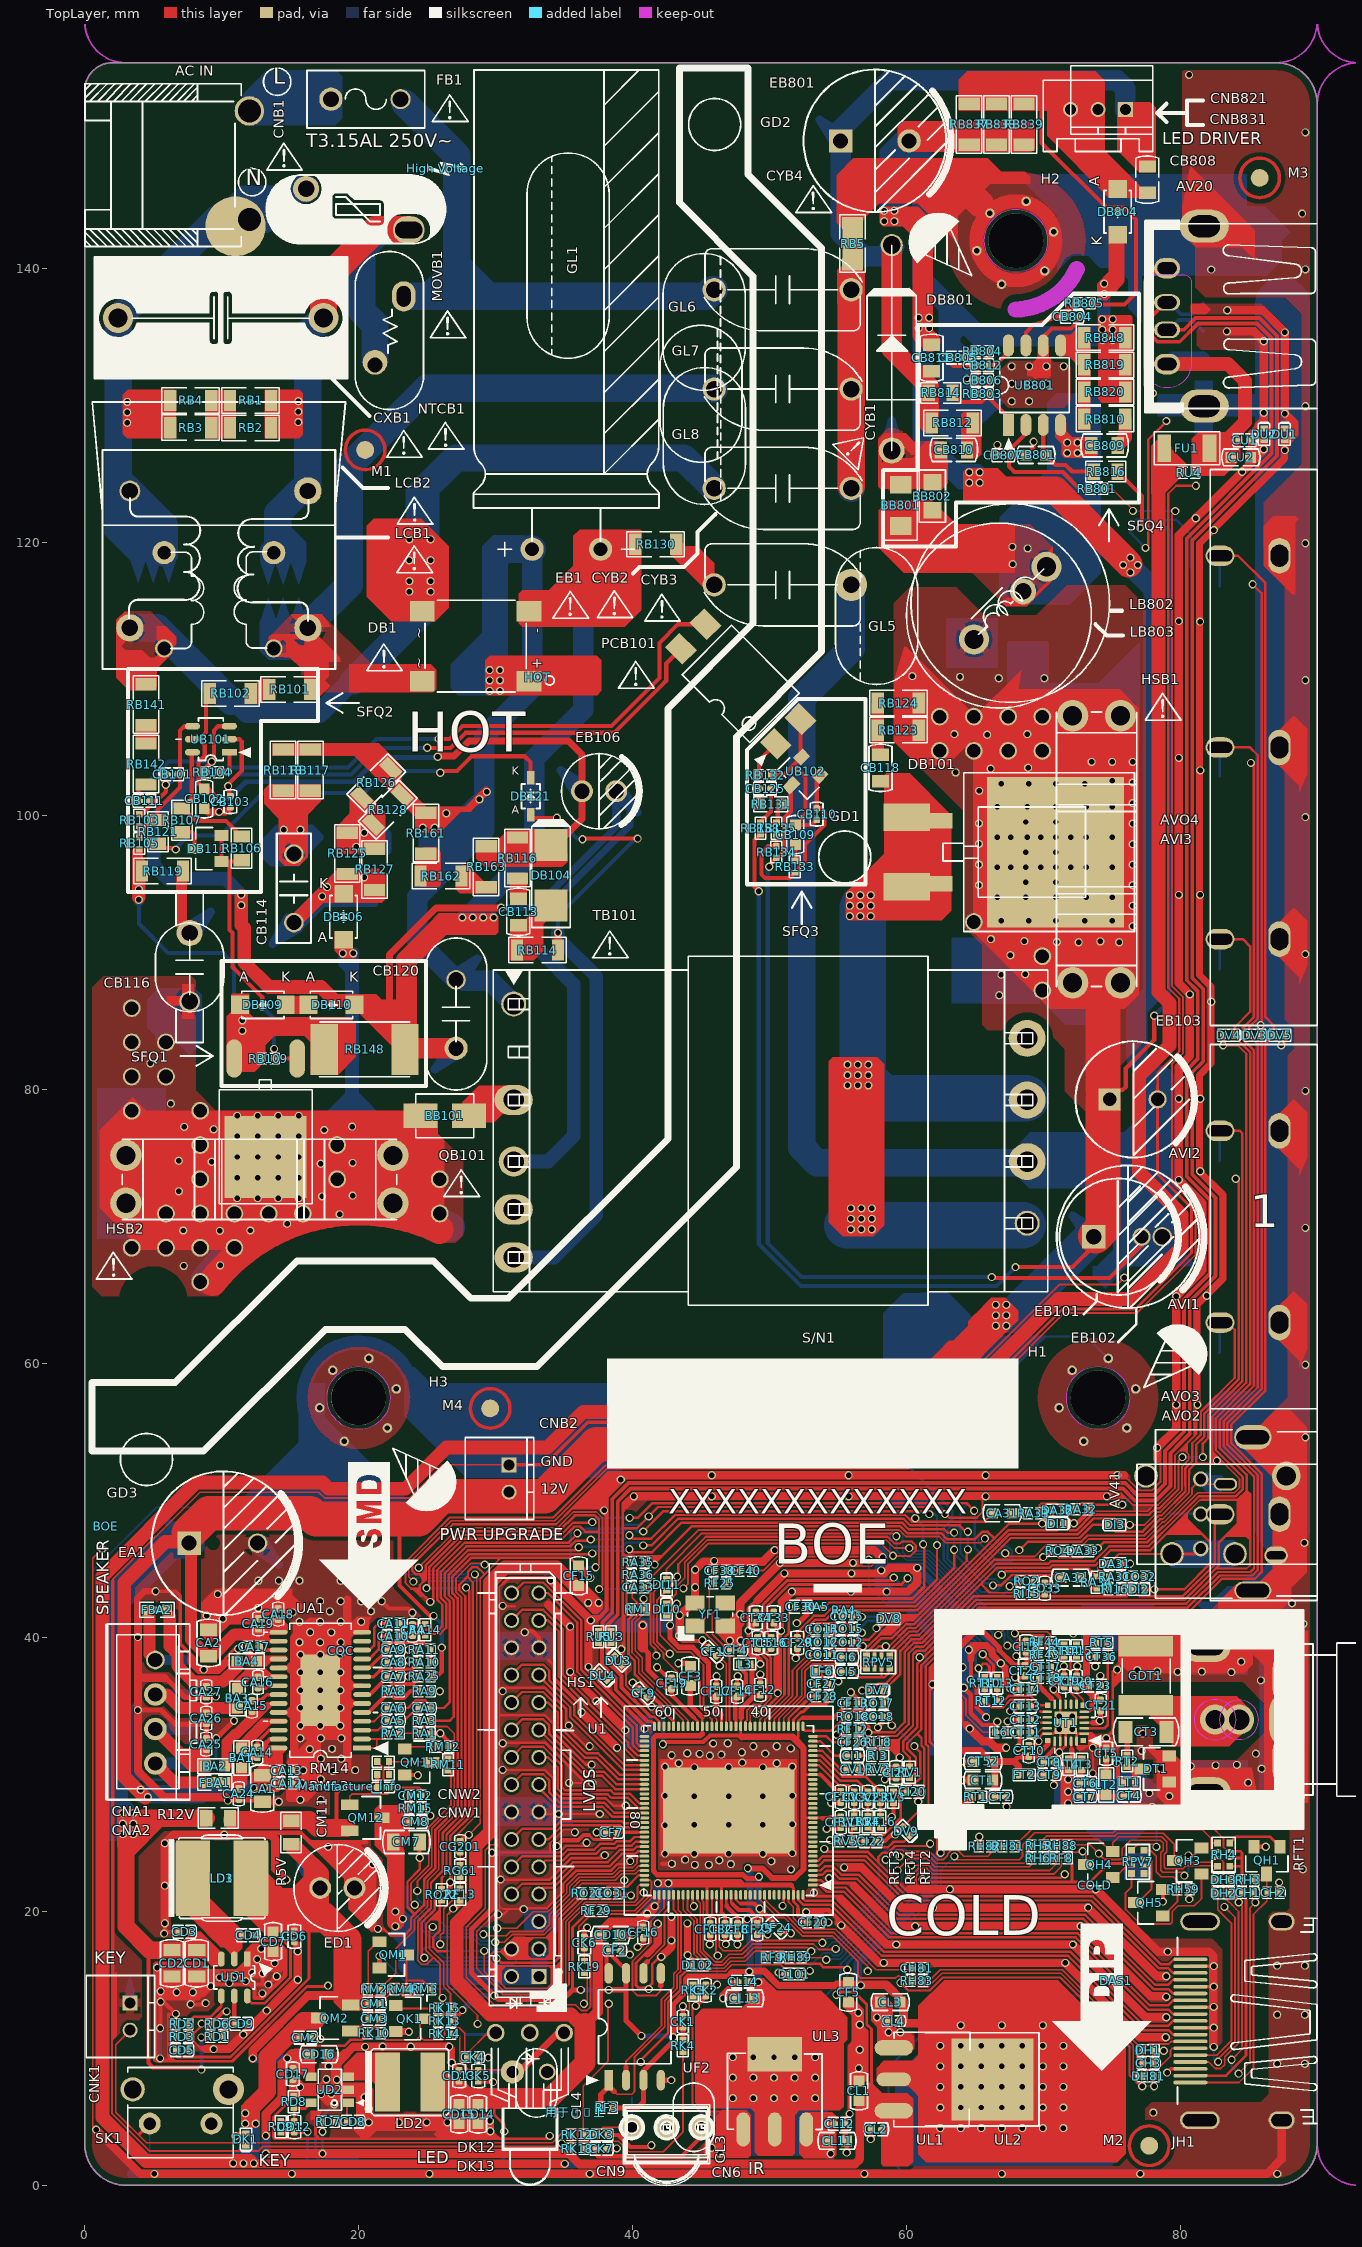
[diagram p0: TopLayer view]
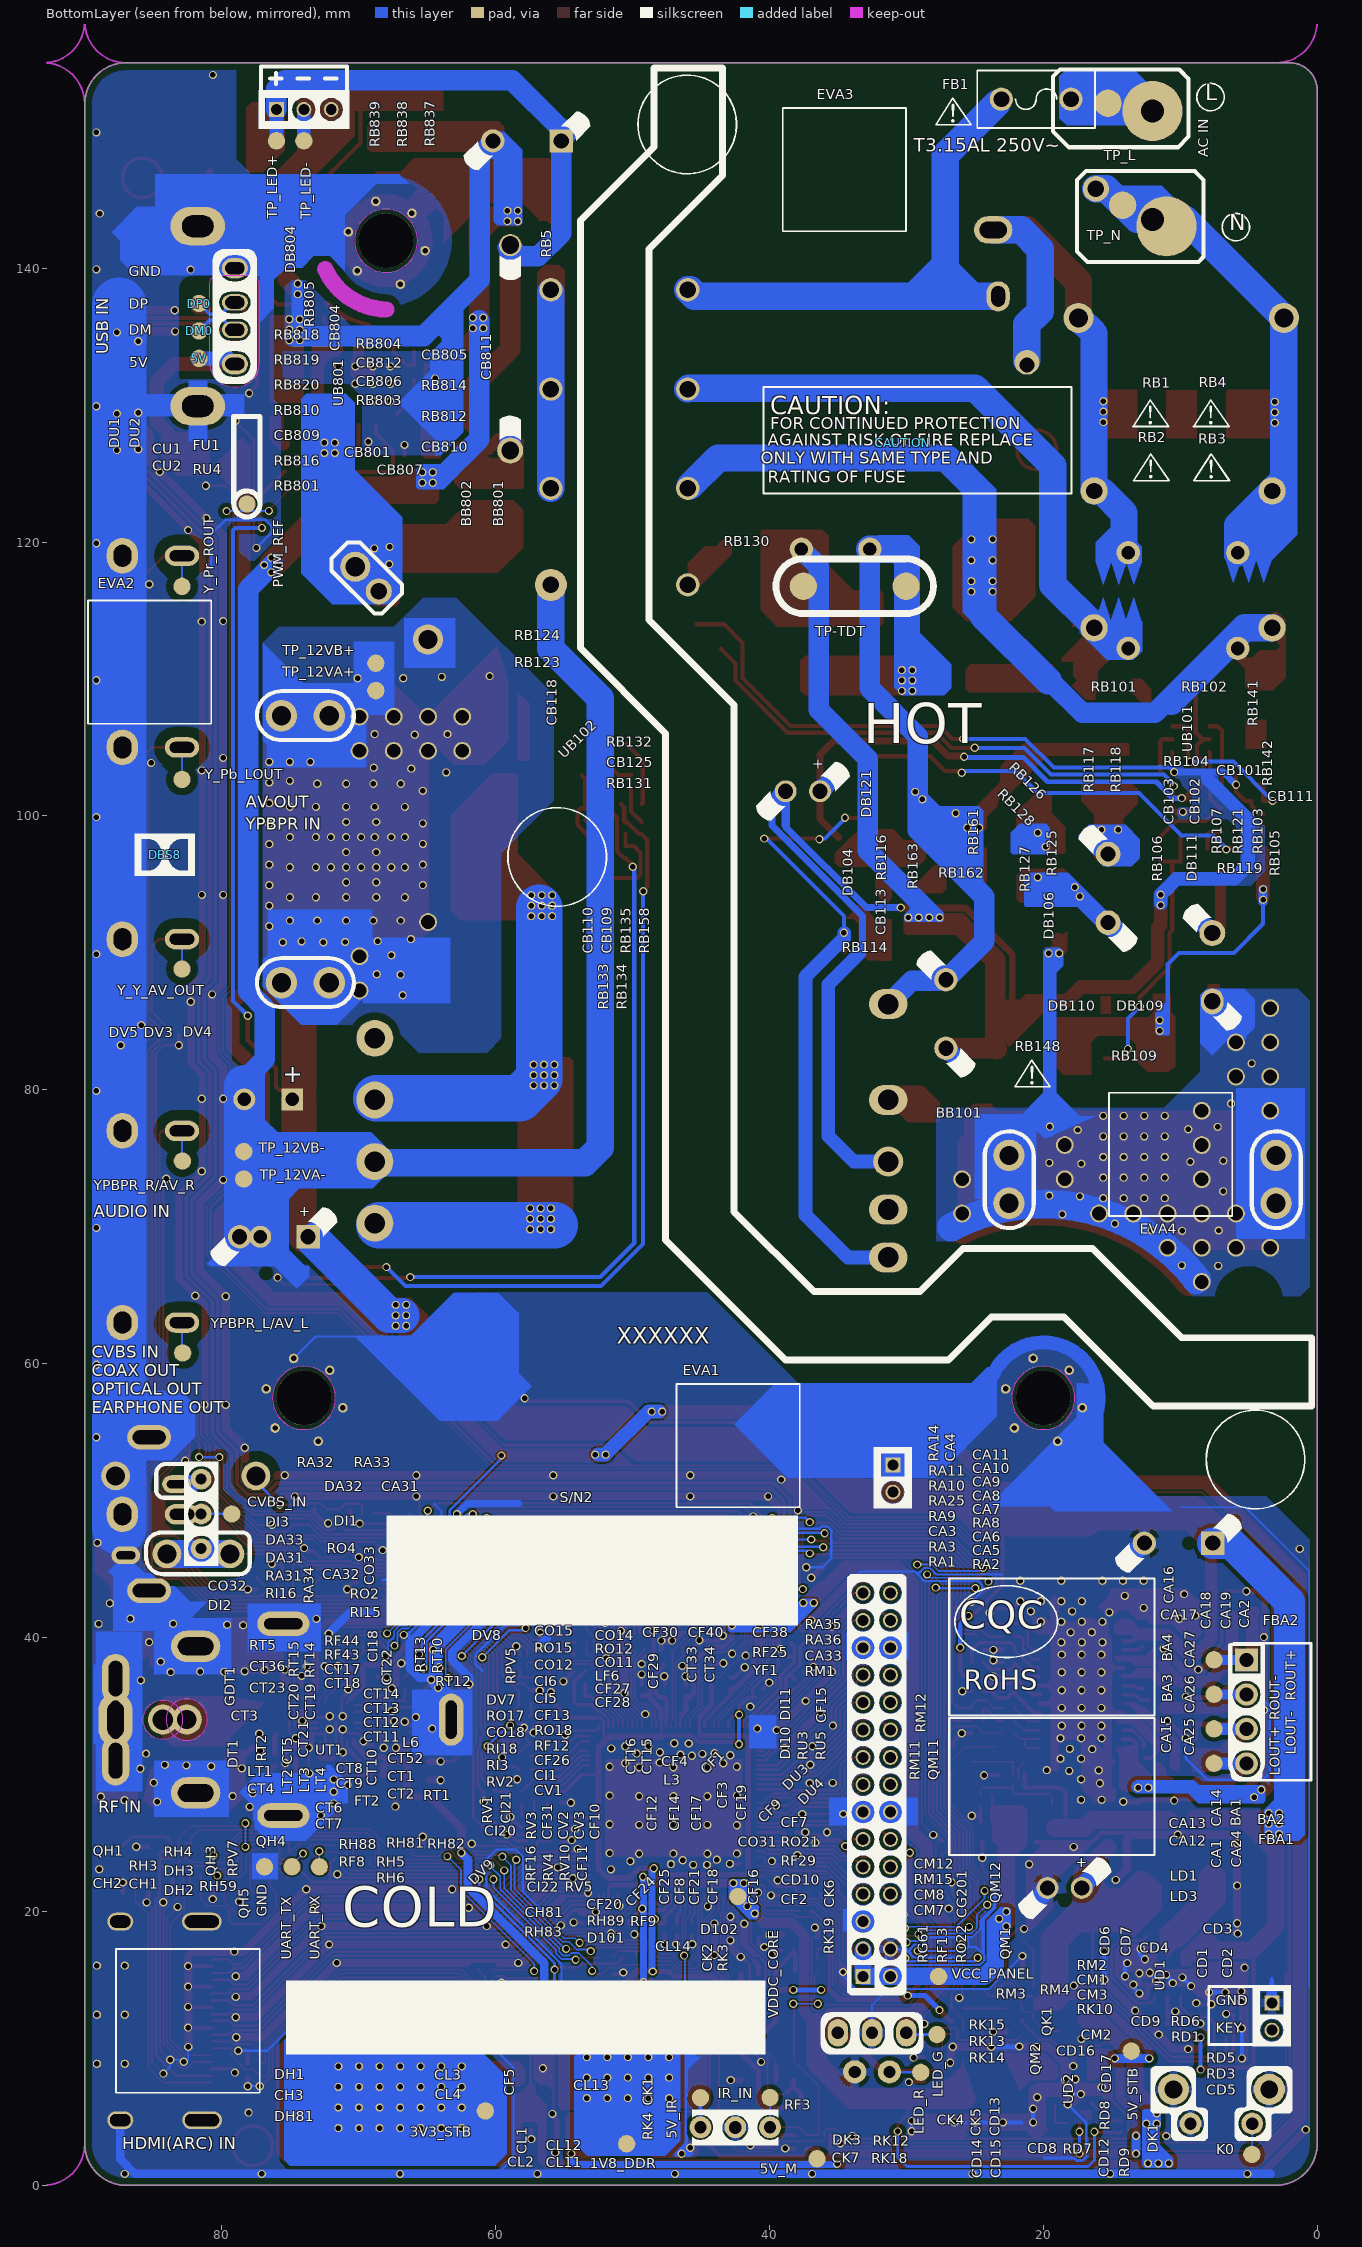
[diagram p1: BottomLayer view, seen from below]
# Altium PCB MISC116569.PcbDoc (part 1 of 15)
Units mm, origin at the board's own origin, x right, y up, seen from the top; angles counter-clockwise.
Board outline 90 x 155 mm, 2 copper layers (TopLayer, BottomLayer), stack 1.571 mm thick; 527 components, 277 nets, 2450 pads, 649 vias.

## Layer stack, top to bottom
TopLayer: signal copper 0.0356
Dielectric: core 1.5, FR-4, Dk 4.8
BottomLayer: signal copper 0.0356

## Board outline
0,3 0,153.003 cw(c2,153.003) 2,155.003 87,155.003 cw(c87,152.003) 90,152.003 90,3 cw(c87,3) 87,0 3,0 cw(c3,3)

## Design rules (kind name [scope] priority, off if disabled: settings)
Clearance ■VIA2VIA_0.41MM [(IsVia OR InPadClass('VIA5')) And Not (IsVia And (AsMM(HoleDiameter) = 0.1)) vs (IsVia OR InPadClass('VIA5')) And Not (IsVia And (AsMM(HoleDiameter) = 0.1))] p1: gap=0.41
Clearance ■KEEPOUT_18mil [(IsTrack Or IsArc) And (AsMM(Width) < 1) And IsKeepOut vs Not IsPad] p2: gap=0.457
Clearance ■HOT_7.2mm [InNetClass('HOT') vs InNetClass('All Nets') And (Not InNetClass('HOT'))] p3: gap=7.2
Clearance ■DFM_NPTH_10mil [(IsPadHoleValid And (PadIsPlated=false) Or IsPad And ((AsMM(PadXSize_AllLayers) < 1) or (AsMM(PadYSize_AllLayers) < 1 )) And IsKeepout) OR HasFootprintPad('ASSE*','0') vs Not IsPad] p4: gap=0.254
Clearance ■DFM_20mil [(IsTrack or IsArc or IsPad) And IsKeepOut vs IsTrack or IsArc or InPoly] p5: gap=0.508
Clearance ■C_RJ45_2mm [InNetClass('RJ45') vs Not InNetClass('RJ45') AND InNet('*')] p6: gap=2
Clearance ■PWR_A12_8mil [((InNetClass('PWR_A12_8mil') or InNet('*12V*') or InNet('*24V*') or InNet('*PVCC*') or InNet('*19V*') or InNet('*AMP*POWER*') or InNet('*AMP*VCC*') or InNet('*LNB*')) And Not InNetClass('A12_8mil_EXC')) and Not IsPad vs Not InPoly] p7: gap=0.203
Clearance ■PS_L2All_3.2mm [InNet('L-1') vs InNet('*')] p8: gap=3.2
Clearance ■PS_L2LN_1.5mm [InNet('L') Or InNet('L-2') Or InNet('L-3') Or InNet('L-4') Or InNet('L-5') Or InNet('L-6') vs InNet('L-N') And Not(InNet('L') Or InNet('L-2') Or InNet('L-3') Or InNet('L-4') Or InNet('L-5') Or InNet('L-6'))] p9: gap=1.5
Clearance ■PS_N2LN_1.5mm [InNet('N') OR InNet('N-1') OR InNet('N-2') OR InNet('N-3') OR InNet('N-4') OR InNet('N-5') OR InNet('N-6') vs InNet('L-N') And Not (InNet('N') OR InNet('N-1') OR InNet('N-2') OR InNet('N-3') OR InNet('N-4') OR InNet('N-5') OR InNet('N-6'))] p10: gap=1.5
Clearance ■PS_L2LN_3.1mm [InNet('L') Or InNet('L-2') Or InNet('L-3') Or InNet('L-4') Or InNet('L-5') Or InNet('L-6') vs InNet('*') And Not (InNet('L-N') Or InNet('L') Or InNet('L-2') Or InNet('L-3') Or InNet('L-4') Or InNet('L-5') Or InNet('L-6') Or OnLayer('KeepOutLayer'))] p11: gap=3.1
Clearance ■PS_N2LN_3.1mm [InNet('N') OR InNet('N-1') OR InNet('N-2') OR InNet('N-3') OR InNet('N-4') OR InNet('N-5') OR InNet('N-6') vs InNet('*') And Not (InNet('L-N') Or InNet('N') OR InNet('N-1') OR InNet('N-2') OR InNet('N-3') OR InNet('N-4') OR InNet('N-5') OR InNet('N-6') Or OnLayer('KeepOutLayer'))] p12: gap=3.1
Clearance ■SIP2GND_8mil [HasFootprint('SIP*') vs InPoly] p13: gap=0.203
Clearance ■C_BGA_0P65 [HasFootprint('BGA*0.65*') vs InPoly] p14: gap=0.127
Clearance ■C_BGA_0P8 [HasFootprint('BGA*0.8*') vs InPoly] p15: gap=0.14
Clearance ■Poly_4mil [InPolygonClass('Poly_4mil') vs Not InPoly] p16: gap=0.102
Clearance ■Poly_5mil [InPolygonClass('Poly_5mil') vs Not InPoly] p17: gap=0.127
Clearance ■Poly_6.2mil [InPolygonClass('Poly_6.2mil') vs Not InPoly] p18: gap=0.157
Clearance ■Poly_8mil [InPolygonClass('Poly_8mil') vs Not InPoly] p19: gap=0.203
Clearance ■C_RFGND_1.8mm [InNet('RFGND') vs Not (InNet('RF*IN*') OR InNet('NetCT28*'))] p20: gap=1.8
Clearance ■ESD_10mil [HasFootprint('*IEC*') Or HasFootprint('*-F1*') Or HasFootprint('ANT-RF*')] p21: gap=0.254
Clearance ■ESD_20mil [HasFootprint('*SHIELD*')] p22: gap=0.508
Clearance ■GND_12mil [InNet('GND') vs InPoly] p23: gap=0.305
Clearance ■ESD_30mil [(HasFootprint('SCART*') OR HasFootprint('AV*') OR HasFootprint('DB15*') OR HasFootprint('PHONE*')) vs OnBottomLayer] p24: gap=0.762
Clearance ■ESD_NT_30mil [HasFootprint('SCART*') Or HasFootprint('PHONE-HD-12') Or HasFootprint('PHONE-HD-17') Or HasFootprint('PHONE-HD-10') Or HasFootprint('PHONE-HD-26') vs InNet('GND') And OnTopLayer] p25: gap=0.762
Clearance ■DFM_TH_5mil [HasFootprint('GND') or HasFootprint('TP*') or HasFootprint('MARK*') or HasFootprint('SPARK_GAP') or HasFootprint('USB-HD-3-2') or HasFootprint('PHONE-HS-20') and Not IsRegion vs OnBottomlayer And IsPad OR IsPadHoleValid] p26: gap=0.127
Clearance ■DFM_HS60_5mil [InPadClass('HS60') vs InPadClass('HS60') OR IsPadHoleValid and not InPadClass('VIA5')] p27: gap=0.127
Clearance ■DFM_BCR_4mm [IsPadHoleValid vs IsBoardCutoutRegion] p28: gap=4
Clearance ■DFM_TH_4mm [OnBottomlayer And IsSMTPin vs IsPadHoleValid and not InPadClass('VIA5')] p29: gap=4
Clearance ■DFM_HS60_4mm [InPadClass('HS60') vs IsPad and OnBottomlayer] p30: gap=4
Clearance ■VIA2VIA_6.2mil [(IsVia OR InPadClass('VIA5')) And Not (IsVia And (AsMM(HoleDiameter) = 0.1)) vs (IsVia OR InPadClass('VIA5')) And Not (IsVia And (AsMM(HoleDiameter) = 0.1))] p31: gap=0.157
Clearance ■VIA2PAD_BGA_5mil [HasFootprint('BGA*') and IsPad vs (IsVia OR InPadClass('VIA5')) And Not (IsVia And (AsMM(HoleDiameter) = 0.1))] p32: gap=0.127
Clearance ■VIA2PAD_6mil [IsVia And Not (IsVia And (AsMM(HoleDiameter) = 0.1)) vs ISPAD and Not HasFootprintPad('*','EPAD') and Not HasFootprintPad('*','257') and Not HasFootprintPad('TP','*') and Not HasFootprintPad('GND','JP*') and Not HasFootprintPad('LQFP216/0.4-2','217') and Not HasFootprintPad('QFP16*','17') and Not HasFootprintPad('QFN16*','17') and Not HasFootprintPad('QFN20*','21') and Not HasFootprintPad('QFN24*','25') and Not HasFootprintPad( 'QFN24*','29') and Not HasFootprintPad('QFN28*','29') and Not HasFootprintPad('QFN32*','33') and Not HasFootprintPad('QFN36*','37') and Not HasFootprintPad('QFN36*','0') and Not HasFootprintPad('QFN32*','0') and Not HasFootprintPad('QFN40*','41') and Not HasFootprintPad('QFN48*','49') and Not HasFootprintPad('LQFP48/0.5-2','49') and Not HasFootprintPad('*SSOP32*','33') and Not HasFootprintPad('SOP8*','9') and Not HasFootprintPad('WSON8/1.27*','9') and Not HasFootprintPad('DFN10/0.5-1*','11') and Not HasFootprintPad('SON16/0.4','9') and Not HasFootprintPad('MSOP10/0.5-1','11') and Not HasFootprintPad('QFN56/0.5','57') and Not HasFootprintPad('LGA31/0.5','3*') and Not InPadClass('VIA_HS60') and Not HasFootprintPad('TSSOP16/0.65-3','17') and Not HasFootprintPad('QFP128/0.5-2','129') and Not HasFootprintPad('QFP128/0.4-5','129') and Not HasFootprintPad('PQFP48*','49') and Not HasFootprintPad('QFP156/0.4-1','157') and Not HasFootprintPad('D2PAK3-TO-252','2') and Not HasFootprintPad('D2PAK3','2')] p33: gap=0.152
Clearance ■PAD2VIA5_6mil [IsPad And ((AsMM(PadXSize_AllLayers) < 2.5) or ((AsMM(PadYSize_AllLayers) < 2.5))) And Not InPadclass('HS60') vs InPadClass('VIA5')] p34: gap=0.152
Clearance "■12mil for Polygon" [InPoly] p35: gap=0.305
Clearance 8mil [All] p36 off: gap=0.203
Clearance 7mil [All] p37 off: gap=0.178
Clearance 6.2mil [All] p38 off: gap=0.157
Clearance 6mil [All] p39 off: gap=0.152
Clearance 5.8mil [All] p40 off: gap=0.147
Clearance 5mil [Not ((IsTrack Or IsArc) And (Layer = 'KeepOutLayer')) vs Not (IsPad or ((IsTrack Or IsArc) And (Layer = 'KeepOutLayer')))] p41 off: gap=0.127
Clearance 4.5mil [Not ((IsTrack Or IsArc) And (Layer = 'KeepOutLayer')) vs Not (IsPad or ((IsTrack Or IsArc) And (Layer = 'KeepOutLayer')))] p42 off: gap=0.114
Clearance "4mil for Minimum" [Not ((IsTrack Or IsArc) And (Layer = 'KeepOutLayer')) vs Not (IsPad or ((IsTrack Or IsArc) And (Layer = 'KeepOutLayer')))] p43: gap=0.102
ComponentClearance ■DFMC_1mm [Not (InComponentClass('Co-Layout') Or HasFootprint('GND')) And (HasFootprint('T/E*') Or HasFootprint('T/PQ*') Or HasFootprint('USB*') Or HasFootprint('HDMI*') Or HasFootprint('USB*') Or HasFootprint('DC-*') Or HasFootprint('AV*') Or HasFootprint('ANT*') Or HasFootprint('PHONE*') Or HasFootprint('CICARD*') Or HasFootprint('CARD*') Or HasFootprint('DVI*') Or HasFootprint('DB*') Or HasFootprint('DP*') Or HasFootprint('DISPLAYPORT*') Or HasFootprint('OPTICAL*') Or HasFootprint('SCART*') Or HasFootprint('RJ45*') Or HasFootprint('USB*') Or HasFootprint('T-*') Or HasFootprint('T/*') Or HasFootprint('200-*') Or HasFootprint('ZhiJia*') Or HasFootprint('Dianpian*') Or HasFootprint('TanPian*') Or HasFootprint('P(*')) vs Not (InComponentClass('Co-Layout') Or HasFootprint('GND'))] p1 off: gap=1 collisioncheckmode=3 verticalgap=1 showdistances=FALSE
ComponentClearance ■DFMC_0.5mm [Not (InComponentClass('Co-Layout') Or HasFootprint('SO-23') Or HasFootprint('DIODE-s0402') Or HasFootprint('GND')) And (HasFootprint('M-*') Or HasFootprint('BGA*') Or HasFootprint('QFP*') Or HasFootprint('QFN*') Or HasFootprint('*DFN*') Or HasFootprint('*SOP*') Or HasFootprint('LGA*') Or HasFootprint('SOIC*') Or HasFootprint('EC*') Or HasFootprint('AC-*') Or HasFootprint('DIODE*') Or HasFootprint('XTAL*') Or HasFootprint('SO-*') Or HasFootprint('L/LC*') Or HasFootprint('L(*') Or HasFootprint('WIFI*') Or HasFootprint('SATA*') Or HasFootprint('POGO*') Or HasFootprint('SOT-223') Or HasFootprint('TO-252') Or HasFootprint('TO-263') Or HasFootprint('KEY*') Or HasFootprint('SW*') Or HasFootprint('DIP*') Or HasFootprint('SIP*') Or HasFootprint('DIP*') Or HasFootprint('CON*') Or HasFootprint('FFC*') Or HasFootprint('FPC*') Or HasFootprint('GDT*') Or HasFootprint('R2512*') Or HasFootprint('R2725*') Or HasFootprint('L2012*') Or HasFootprint('L2520*')) vs Not (InComponentClass('Co-Layout') Or HasFootprint('SO-23') Or HasFootprint('DIODE-s0402') Or HasFootprint('GND'))] p2 off: gap=0.5 collisioncheckmode=3 verticalgap=0.5 showdistances=FALSE
ComponentClearance ■DFMC_0.4mm [Not (InComponentClass('Co-Layout') Or HasFootprint('GND')) And (HasFootprint('C0201*') Or HasFootprint('C0402*') Or HasFootprint('C0603*') Or HasFootprint('C0805*') Or HasFootprint('C1206*') Or HasFootprint('C1210*') Or HasFootprint('R0201*') Or HasFootprint('R0402*') Or HasFootprint('R0603*') Or HasFootprint('R0805*') Or HasFootprint('R*0402*') Or HasFootprint('L0201*') Or HasFootprint('L0402*') Or HasFootprint('L0603*') Or HasFootprint('L0805*') Or HasFootprint('L1206*') Or HasFootprint('DIODE-s0402')) vs Not (InComponentClass('Co-Layout') Or HasFootprint('GND')) And (HasFootprint('C0201*') Or HasFootprint('C0402*') Or HasFootprint('C0603*') Or HasFootprint('C0805*') Or HasFootprint('C1206*') Or HasFootprint('C1210*') Or HasFootprint('R0201*') Or HasFootprint('R0402*') Or HasFootprint('R0603*') Or HasFootprint('R0805*') Or HasFootprint('R*0402*') Or HasFootprint('L0201*') Or HasFootprint('L0402*') Or HasFootprint('L0603*') Or HasFootprint('L0805*') Or HasFootprint('L1206*') Or HasFootprint('DIODE-s0402'))] p3 off: gap=0.4 collisioncheckmode=3 verticalgap=0.4 showdistances=FALSE
ComponentClearance ■DFMC_0.36mm [Not (InComponentClass('Co-Layout') Or HasFootprint('GND')) And HasFootprint('R1206*') vs Not (InComponentClass('Co-Layout') Or HasFootprint('GND')) And HasFootprint('R1206*')] p4 off: gap=0.36 collisioncheckmode=3 verticalgap=0.36 showdistances=FALSE
ComponentClearance ■DFMC_0.25mm [Not (InComponentClass('Co-Layout') Or HasFootprint('GND')) vs Not (InComponentClass('Co-Layout') Or HasFootprint('GND'))] p5 off: gap=0.25 collisioncheckmode=3 verticalgap=0.25 showdistances=FALSE
DiffPairsRouting ■DiffPair_USB_DiffPairsRouting [InDifferentialPairClass('USB')] p1: maxlimit=0.127 minlimit=0.102 mostfreqgap=0.127 maxuncoupledlength=5.08
DiffPairsRouting ■DiffPair_LVDS_DiffPairsRouting [InDifferentialPairClass('LVDS')] p2: maxlimit=0.127 minlimit=0.102 mostfreqgap=0.127 maxuncoupledlength=12.7
DiffPairsRouting ■DiffPair_HDMI_DiffPairsRouting [InDifferentialPairClass('HDMI')] p3: maxlimit=0.127 minlimit=0.102 mostfreqgap=0.127 maxuncoupledlength=5.08
DiffPairsRouting [All] p4: maxlimit=0.254 minlimit=0.254 mostfreqgap=0.254 maxuncoupledlength=12.7
FabricationTestPointUsage TestPointUsage [All] p1: valid=0 allowmultiple=FALSE
FabricationTestpoint Testpoint [All] p1: side=3 testpointundercomponent=TRUE minsize=1.016 maxsize=2.54 preferedsize=1.524 minholesize=0.508 maxholesize=1.016 preferedholesize=0.813 testpointgrid=0.025 allowsidetop=TRUE allowsidebottom=TRUE usegrid=TRUE gridtolerance=0
HoleSize HoleSize_VIA [ISVIA] p1 off: absolutevalues=TRUE maxlimit=0.6 minlimit=0.2 maxpercent=80.000 minpercent=20.000
HoleToHoleClearance Hole2Hole [All] p1 off: gap=0.457 allowstackedmicrovias=FALSE
MatchedLengths DiffPair_USB_MatchedLengths [InDifferentialPairClass('USB')] p1: tolerance=2.54 checknetsindiffpair=TRUE checkdiffpairvsdiffpair=TRUE checkothers=TRUE
MatchedLengths DiffPair_LVDS_MatchedLengths [InDifferentialPairClass('LVDS')] p2: tolerance=2.54 checknetsindiffpair=TRUE checkdiffpairvsdiffpair=TRUE checkothers=TRUE
MatchedLengths DiffPair_HDMI_MatchedLengths [InDifferentialPairClass('HDMI')] p3: tolerance=2.54 checknetsindiffpair=TRUE checkdiffpairvsdiffpair=TRUE checkothers=TRUE
MinimumAnnularRing [All] p1: minimumring=0.1
MinimumSolderMaskSliver ■MiniSolderMaskSliver [All] p1 off: minsoldermaskwidth=0.098
NetAntennae [Not (HasFootprint('ANT-7') or HasFootprint('ANT-BLUECORE'))] p1: netantennaetolerance=1.016
PermittedLayers [All] p1: toplayerpermitted=TRUE bottomlayerpermitted=TRUE
PlaneClearance ■Plane_ESD_30mil [(HasFootprint('SCART*') OR HasFootprint('AV*') OR HasFootprint('DB15*') OR HasFootprint('PHONE*'))] p1: clearance=0.762
PlaneClearance ■Plane_All_9mil [All] p2: clearance=0.229
PlaneConnect ■PlaneOverAll [IsVia or InPadClass('VIA5') Or HasFootprint('ASSE*') OR InPadclass('HS60')] p1: planeconnectstyle=Direct reliefexpansion=0.508 reliefentries=4 reliefconductorwidth=0.254 reliefairgap=0.254
PlaneConnect ■PlaneConnect [All] p2: planeconnectstyle=Relief reliefexpansion=0.305 reliefentries=4 reliefconductorwidth=0.762 reliefairgap=0.305
PolygonConnect ■PourOverAll [IsVia Or InPadclass('HS60') Or InPadClass('VIA5') Or HasFootprint('ASSE*') Or HasFootprint('DIODE-S0402') Or HasFootprint('RCL0524P') Or HasFootprint('SOT-89') OR HasFootprint('SOT-223') OR HasFootprint('TO-252') OR HasFootprint('TO-263') OR HasFootprint('DIODE') OR HasFootprint('SW-HS-2') OR HasFootprint('HDMI*') OR HasFootprint('SO-8B') OR HasFootprint('GND') OR HasFootprint('PHONE*') OR HasFootprint('DIP18/2.54-2') OR HasFootprint('DIP18/2.54-1') OR HasFootprint('UFL-R-SMT-1') OR HasFootprint('WIFI') OR HasFootprint('UM02BS') OR HasFootprint('*SCART*') OR HasFootprint('TSOT23-8/0.65') OR HasFootprint('*SOT-23-*') OR HasFootprint('SOP23-5-1') OR HasFootprint('SOP6/0.95') OR HasFootprint('M-WIFI-2-M603USA1') OR HasFootprint('M-MT7632U') OR HasFootprint('SOP8/1.27') OR HasFootprint('SOP8/1.27-3') vs IsPolygon] p1: connectstyle=Direct reliefconductorwidth=0.254 reliefentries=4 polygonreliefangle="90 Angle"
PolygonConnect ■BGA_0P65 [HasFootprint('BGA*0.65*') vs IsPoly] p2: connectstyle=Relief reliefconductorwidth=0.203 reliefentries=4 polygonreliefangle="45 Angle"
PolygonConnect ■BGA_0P8 [HasFootprint('BGA*0.8*') vs IsPoly] p3: connectstyle=Relief reliefconductorwidth=0.229 reliefentries=4 polygonreliefangle="45 Angle"
PolygonConnect ■Polygon_RFGND [InNet('RFGND')] p4: connectstyle=Direct reliefconductorwidth=0.254 reliefentries=4 polygonreliefangle="90 Angle"
PolygonConnect ■ESD_SCART [HasFootprint('SCART*') vs IsPolygon And onBottomlayer] p5: connectstyle=Direct reliefconductorwidth=0.762 reliefentries=4 polygonreliefangle="90 Angle"
PolygonConnect ■C2Polygon_35mil [HasFootprint('EC*') vs IsPolygon] p6: connectstyle=Relief reliefconductorwidth=0.889 reliefentries=4 polygonreliefangle="90 Angle"
PolygonConnect ■C2Polygon_30mil [(HasFootprint('*0805*') OR HasFootprint('*1206*')) vs IsPolygon] p7: connectstyle=Relief reliefconductorwidth=0.762 reliefentries=4 polygonreliefangle="90 Angle"
PolygonConnect ■C2Polygon_25mil [HasFootprint('*0603*') Or IsThruPin vs IsPolygon] p8: connectstyle=Relief reliefconductorwidth=0.635 reliefentries=4 polygonreliefangle="90 Angle"
PolygonConnect ■C2Polygon_12mil [IsSMTPin vs IsPolygon] p9: connectstyle=Relief reliefconductorwidth=0.305 reliefentries=4 polygonreliefangle="90 Angle"
RoutingVias 0.6_0.4 [All] p1: holewidth=0.4 width=0.6 viastyle="Through Hole" minholewidth=0.4 minwidth=0.6 maxholewidth=0.4 maxwidth=0.6
RoutingVias 0.8_0.5 [All] p2 off: holewidth=0.5 width=0.8 viastyle="Through Hole" minholewidth=0.5 minwidth=0.8 maxholewidth=0.5 maxwidth=0.8
RoutingVias 0.5_0.3 [All] p3 off: holewidth=0.3 width=0.5 viastyle="Through Hole" minholewidth=0.3 minwidth=0.5 maxholewidth=0.3 maxwidth=0.5
RoutingVias 0.45_0.25 [All] p4 off: holewidth=0.25 width=0.45 viastyle="Through Hole" minholewidth=0.25 minwidth=0.45 maxholewidth=0.25 maxwidth=0.45
RoutingVias 0.4_0.2 [All] p5 off: holewidth=0.2 width=0.4 viastyle="Through Hole" minholewidth=0.2 minwidth=0.4 maxholewidth=0.2 maxwidth=0.4
RoutingVias 0.25_0.1 [All] p6 off: holewidth=0.1 width=0.25 viastyle="Through Hole" minholewidth=0.1 minwidth=0.25 maxholewidth=0.1 maxwidth=0.25
SMDNeckDown ■SMDNeckDown_Chip [HasFootprint('FFC*') or HasFootprint('QFP*') or HasFootprint('QFN*') or HasFootprint('HDMI*') or HasFootprint('BGA*')] p1: percent=100.000
SMDToCorner [All] p1 off: distance=40000
ShortCircuit ■ShortCircuit_ViaOnEpad [HasFootprintPad( '*','EPAD') vs IsVia AND InNet('*')] p1: allowed=TRUE
ShortCircuit ■ShortCircuit_JP [HasFootprintPad( 'GND','JP_1K') vs HasFootprintPad( 'GND','JP_2K')] p2: allowed=TRUE
ShortCircuit ■ShortCircuit_0402 [HasFootprintPad('R0402SC','1') OR HasFootprintPad('R0402SC','2') vs HasFootprintPad('R0402SC','3')] p3: allowed=TRUE
ShortCircuit ■ShortCircuit_0603 [HasFootprintPad('R0603SC','1') OR HasFootprintPad('R0603SC','2') vs HasFootprintPad('R0603SC','3')] p4: allowed=TRUE
ShortCircuit ■ShortCircuit_0805 [HasFootprintPad('R0805SC','1') OR HasFootprintPad('R0805SC','2') vs HasFootprintPad('R0805SC','3')] p5: allowed=TRUE
ShortCircuit ■ShortCircuit_1206 [HasFootprintPad('R1206SC','1') OR HasFootprintPad('R1206SC','2') vs HasFootprintPad('R1206SC','3')] p6: allowed=TRUE
ShortCircuit ■ShortCircuit [InNet('*')] p7: allowed=FALSE
SilkToSilkClearance ■Silk2Silk [All] p1: silktosilkclearance=0.127
SilkscreenOverComponentPads ■SilkOverPads [IsText] p1: minsilkscreentomaskgap=0.003
SolderMaskExpansion ■SolderMask_VIA [IsVia] p1: expansion=0.13
SolderMaskExpansion ■SolderMask_All [All] p2: expansion=0.051
UnRoutedNet ■UnRoutedNet [All] p1:
ViasUnderSMD [All] p1: allowed=FALSE
Width ■Width_2.5mm [InFromToClass('Width_2.5mm')] p1: maxlimit=2.5 minlimit=2.5 preferedwidth=2.5
Width ■Width_1.5mm [InFromToClass('Width_1.5mm')] p2: maxlimit=1.5 minlimit=1.5 preferedwidth=1.5
Width ■DiffPair_USB_Width [InDifferentialPairClass('USB')] p3: maxlimit=0.279 minlimit=0.102 preferedwidth=0.279
Width ■DiffPair_LVDS_Width [InDifferentialPairClass('LVDS')] p4: maxlimit=0.178 minlimit=0.102 preferedwidth=0.178
Width ■DiffPair_HDMI_Width [InDifferentialPairClass('HDMI')] p5: maxlimit=0.178 minlimit=0.102 preferedwidth=0.178
Width [All] p6: maxlimit=12.7 minlimit=0.076 preferedwidth=0.203
14 further rules are at their usual default settings.

## Classes and differential pairs
net class POWER: 12V 12V-COIL 12V_OVP BRO D_QB101 DRIM GND L L5 L-1 L-2 L-3 L-5 L-N LED+ LED_FB LED_OVP N-2 N-3 NetBB101_2 NetBB801_2 NetCB101_1 NetCB102_1 NetCB103_2 NetCB109_1 NetCB109_2 NetCB110_2 NetCB111_1 NetCB113_1 NetCB113_2 NetCB114_1 NetCB116_1 NetCB118_2 NetCB125_1 NetCB125_2 NetCB801_1 NetCB804_2 NetCB805_1 NetCB807_2 NetCB809_1 NetCB810_2 NetCB812_1 NetCYB1_2 NetCYB3_1 NetCYB4_2 NetDB109_A NetDB109_K NetDB111_1 NetDB111_2 NetDB121_K NetRB106_1 NetRB141_1 NetRB161_2 NetRB162_2 NetRB810_1 PWM_REF SGND SNB-D- SNB-RM VBRIDGE VSTR
net class HOT: 12V_OVP BRO D_QB101 L L5 L-1 L-2 L-3 L-5 L-N N-2 N-3 NetBB101_2 NetCB101_1 NetCB102_1 NetCB103_2 NetCB111_1 NetCB113_1 NetCB113_2 NetCB114_1 NetCB116_1 NetCYB3_1 NetDB109_A NetDB109_K NetDB111_1 NetDB111_2 NetDB121_K NetRB106_1 NetRB141_1 NetRB161_2 NetRB162_2 SGND SNB-D- SNB-RM VBRIDGE VSTR
component class TV#08_Tuner: CT1 CT2 CT3 CT4 CT5 CT6 CT7 CT8 CT9 CT10 CT11 CT12 CT13 CT14 CT15 CT16 CT17 CT18 CT19 CT20 CT21 CT22 CT23 CT33 CT34 CT36 CT52 DT1 FT2 GDT1 LT1 LT2 LT3 LT4 RFT1 RFT2 RFT3 RFT4 RT1 RT2 RT5 RT10 RT12 RT13 RT14 RT15 UT1
component class TV#07_AMP: BA1 BA2 BA3 BA4 CA1 CA2 CA3 CA4 CA5 CA6 CA7 CA8 CA9 CA10 CA11 CA12 CA13 CA14 CA15 CA16 CA17 CA18 CA19 CA24 CA25 CA26 CA27 CNA1 CNA2 EA1 FBA1 FBA2 LOUT+ LOUT- RA1 RA2 RA3 RA4 RA5 RA8 RA9 RA10 RA11 RA14 RA25 ROUT+ ROUT- UA1
component class TV#06_HDMI: CH1 CH2 CH3 CH81 DH1 DH2 DH3 DH81 GND JH1 QH1 QH3 QH4 QH5 RH3 RH4 RH5 RH6 RH59 RH81 RH82 RH83 RH88 RH89 RPV7 UART_RX UART_TX
component class TV#05_AV&YPBPR&COAX&OPTICAL&USB: 5V AV20 AV41 AVI1 AVI2 AVI3 AVO2 AVO3 AVO4 CA31 CA32 CA33 CI1 CI5 CI6 CI20 CI21 CI22 CO11 CO12 CO14 CO15 CO18 CO31 CO32 CO33 CU1 CU2 CV1 CV2 CV3 CVBS_IN DA31 DA32 DA33 DI1 DI2 DI3 DM0 DP0 DU1 DU2 DU3 DU4 DV3 DV4 DV5 DV7 DV8 DV9 FU1 RA31 RA32 RA33 RA34 RA35 RA36 RI3 RI15 RI16 RI18 RO2 RO4 RO12 RO15 RO17 RO18 RO21 RO22 RPV5 RU3 RU4 RU5 RV1 RV2 RV3 RV4 RV5 RV10 Y_Pb_LOUT Y_Pr_ROUT Y_Y_AV_OUT YPBPR_L/AV_L YPBPR_R/AV_R
component class TV#04_LVDS: CM7 CM8 CM11 CM12 CNW1 CNW2 QM11 QM12 R5V R12V RM11 RM12 RM13 RM14 RM15 VCC_PANEL
component class TV#03_IR&KEY: 5V_IR CK1 CK2 CK4 CK5 CK6 CK7 CN6 CN9 CNK1 DK1 DK3 DK12 DK13 GL3 GL4 GL7 GL8 IR_IN K0 LED_G LED_R QK1 RK3 RK4 RK10 RK12 RK13 RK14 RK15 RK18 RK19 SK1
component class TV#02_V53: CF1 CF2 CF3 CF4 CF5 CF7 CF8 CF9 CF10 CF11 CF12 CF13 CF14 CF15 CF16 CF17 CF18 CF19 CF20 CF21 CF24 CF25 CF26 CF27 CF28 CF29 CF30 CF31 CF38 CF40 CI18 D101 D102 DI10 DI11 L3 L6 LF6 RF3 RF8 RF9 RF12 RF13 RF16 RF25 RF29 RF43 RF44 U1 UF2 YF1
component class TV#01_POWER: 1V8_DDR 3V3_STB 5V_M 5V_STB CD1 CD2 CD3 CD4 CD5 CD6 CD7 CD8 CD9 CD10 CD12 CD13 CD14 CD15 CD16 CD17 CG201 CL1 CL2 CL3 CL4 CL11 CL12 CL13 CL14 CM1 CM2 CM3 ED1 LD1 LD2 LD3 QM1 QM2 RD1 RD3 RD5 RD6 RD7 RD8 RD9 RG61 RM1 RM2 RM3 RM4 UD1 UD2 UL1 UL2 UL3 VDDC_CORE
component class SCH_info: BOE DBS8 DBSR HS1 HS2 XXXXXX XXXXXXXXXXXXX XXXXXZ 用于U1上
component class PS#01_XXXXXXXXXXXXX: BB101 BB801 BB802 CB101 CB102 CB103 CB109 CB110 CB111 CB113 CB114 CB116 CB118 CB120 CB125 CB801 CB804 CB805 CB806 CB807 CB808 CB809 CB810 CB811 CB812 CNB1 CNB2 CNB821 CNB831 "Conformal Coating" CXB1 CYB1 CYB2 CYB3 CYB4 DB1 DB101 DB104 DB106 DB109 DB110 DB111 DB121 DB801 DB804 EB1 EB101 EB102 EB103 EB106 EB801 EVA1 EVA2 EVA3 EVA4 FB1 GD1 GD2 GD3 GL1 GL5 GL6 GL7 GL8 HSB1 HSB2 LB802 LB803 LCB1 LCB2 ML1 MOVB1 NTCB1 PCB101 PWM_REF QB101 RB1 RB2 RB3 RB4 RB5 RB101 RB102 RB103 RB104 RB105 RB106 RB107 RB109 RB114 RB116 RB117 RB118 RB119 RB121 RB123 RB124 RB125 RB126 RB127 RB128 RB130 RB131 RB132 RB133 RB134 RB135 RB141 RB142 RB148 RB158 RB161 RB162 RB163 RB801 RB803 RB804 RB805 RB810 RB812 RB814 RB816 RB818 RB819 RB820 RB837 RB838 RB839 SFQ1 SFQ2 SFQ3 SFQ4 TB101 TP-TDT TP_12VA+ TP_12VA- TP_12VB+ TP_12VB- TP_L TP_LED+ TP_LED- TP_N UB101 UB102 UB801
component class PCB_info: CAUTION COLD CQC DAS1 H1 H2 H3 H4 "High Voltage" HOT M1 M2 M3 M4 Manufacture_Info S/N1 S/N2
polygon class Poly_5mil: 5
pad class HS60: Free-HS60
pad class VIA5: Free-VIA5 Free-via5

## Components (designator, comment, footprint, x,y, rotation, side; value= is the part's Value field where it differs from the comment)
1V8_DDR "TEST" TP 50.427,3.025 r180 bottom
3V3_STB "TEST" TP 60.748,5.428 r0 bottom
5V "DM0" TP 81.656,133.417 r180 bottom
5V_IR "TEST  SL" TP 45.042,6.391 r180 bottom
5V_M "TEST" TP 36.52,1.93 r180 bottom
5V_STB "TEST" TP 13.571,9.792 r180 bottom
AV20 "USB jack,USB Jack,H,Single,flange,DIP,WLUS-050F USB,WLCO" USB1-HD-2 91.997,136.5 r90 top locked
AV41 "NC/Earphone jack,Earphone Jack,H,Φ3.5,CH7.0,Black,switch,Seal,DIP,PJ-373A,JSL" PHONE-HD-42 90,49 r90 top locked
AVI1 "RCA jack,RCA Jack,AV3,H,Yellow、White、Red,CH5.5,D14,Seal,DIP,AV3-8.4-15C,JSL (MI material)" AV3-H14-15 90,63 r90 top locked
AVI2 "NC/RCA jack,RCA Jack,AV2,H,White、Red,CH5.5,D14,Seal,DIP,AV63-02S-0030,QS (MI hand-insert material)" AV2-H14-15 90,70 r90 top locked
AVI3 "RCA jack,RCA Jack,AV3,H,Green、Blue、Red,CH5.5,D14,Seal,DIP,AV3-8.4-15C,JSL" AV3-H14-15 90,105 r90 top locked
AVO2 "NC/Optical jack,OPTICAL,H,DIP,DQT-026D-2,DQ" OPTICAL-HD-3 90,49.025 r90 top locked
AVO3 "NC/RCA jack,RCA Jack,AV3,H,Orange、White、Red,CH5.5,D14,Seal,DIP,AV3-8.4-15C,JSL" AV3-H14-15 90,63 r90 top locked
AVO4 "NC/RCA jack,RCA Jack,AV3,H,Yellow、White、Red,CH5.5,D14,Seal,DIP,RC075-F03L3BY-A,YUQIU (MI material)" AV3-H14-15 90,105 r90 top locked
BA1 "Ferrite bead,BEAD,600ohm,0603,2A,SMD,TP,EPZ1608E601-2R0TF,Sunlord" L0603 11.443,31.204 r270 top
BA2 "Ferrite bead,BEAD,600ohm,0603,2A,SMD,TP,EPZ1608E601-2R0TF,Sunlord" L0603 9.5,30.607 r180 top
BA3 "Ferrite bead,BEAD,600ohm,0603,2A,SMD,TP,EPZ1608E601-2R0TF,Sunlord" L0603 11.151,35.547 r270 top
BA4 "Ferrite bead,BEAD,600ohm,0603,2A,SMD,TP,EPZ1608E601-2R0TF,Sunlord" L0603 11.832,38.265 r180 top
BB101 "Ferrite bead,BEAD,50ohm,3.0×4.0,9A,SMD,TP,SMB-302540-K5B-L1,SOLDIER" L(4*3*2.55)-S 26.289,78.092 r0 top
BB801 "Ferrite bead,BEAD,60ohm@100MHz,1206,4A,SMD,TP,PZ3216U600-4R0TF,Sunlord" L1206 59.589,122.682 r90 top
BB802 "Ferrite bead,BEAD,600ohm±25%,0805,2000mA,SMD,TP,UPZ2012E601-2R0TF,Sunlord" L0805 61.9,123.355 r90 top
BOE "PCB_NAME2" PCB_NAME 1.529,48.138 r90 top
CA1 "10uF-0805-X5R-±20%-16V" C0805 12.967,28.969 r90 top
CA2 "NC/10uF-0805-X5R-±20%-16V" C0805 9.03,39.599 r270 top
CA3 "3300pF-0402-X7R-±10%-50V" C0402#1 24.804,34.849 r180 top
CA4 "3300pF-0402-X7R-±10%-50V" C0402#1 23.935,40.538 r270 top